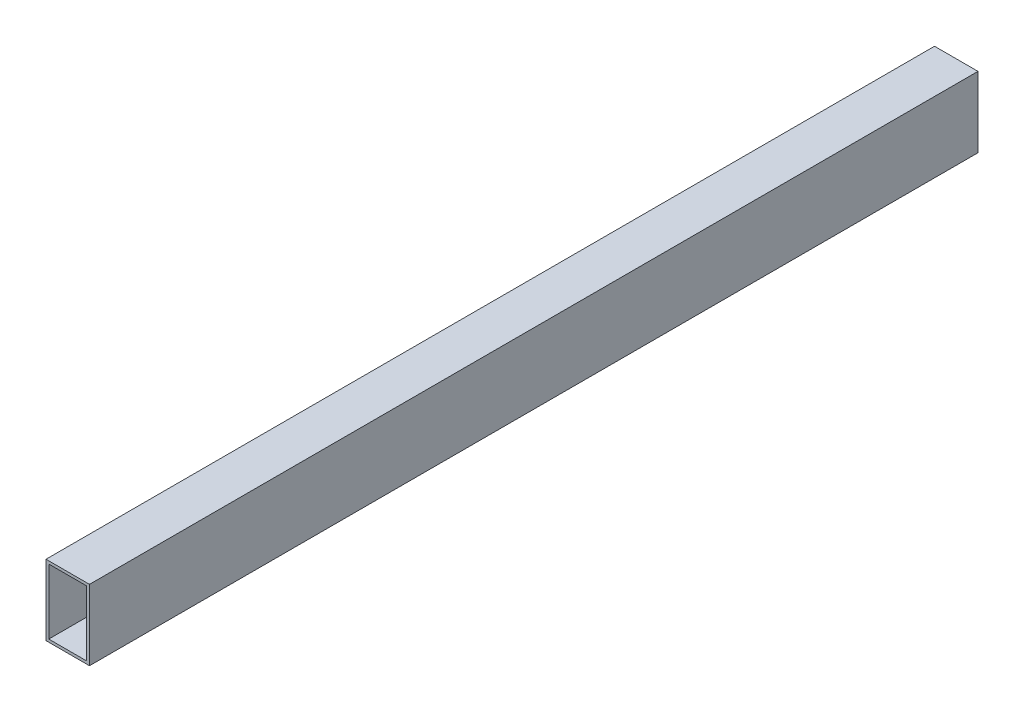
SolidWorks part; units mm, degrees
ref_plane "Front Plane" through (0, 0, 0) normal (0, 0, 1) x (1, 0, 0)
ref_plane "Top Plane" through (0, 0, 0) normal (0, 1, 0) x (1, 0, 0)
ref_plane "Right Plane" through (0, 0, 0) normal (1, 0, 0) x (0, 0, -1)
sketch "Sketch1" plane through (0, 0, 0) normal (0, 0, 1) x (1, 0, 0)
  line L0 (-50.9894, 24.8251) -> (-78.505, 24.8251)
  line L1 (-48.9894, 26.8251) -> (-80.505, 26.8251)
  line L2 (-48.9894, 26.8251) -> (-48.9894, -24.2841)
  line L3 (-48.9894, -24.2841) -> (-80.505, -24.2841)
  line L4 (-80.505, 26.8251) -> (-80.505, -24.2841)
  line L5 (-78.505, 24.8251) -> (-78.505, -22.2841)
  line L6 (-50.9894, -22.2841) -> (-78.505, -22.2841)
  line L7 (-50.9894, 24.8251) -> (-50.9894, -22.2841)
  dimension "D1" = 2
extrude "Boss-Extrude1" add sketch "Sketch1" along normal up to surface (644 mm away)
